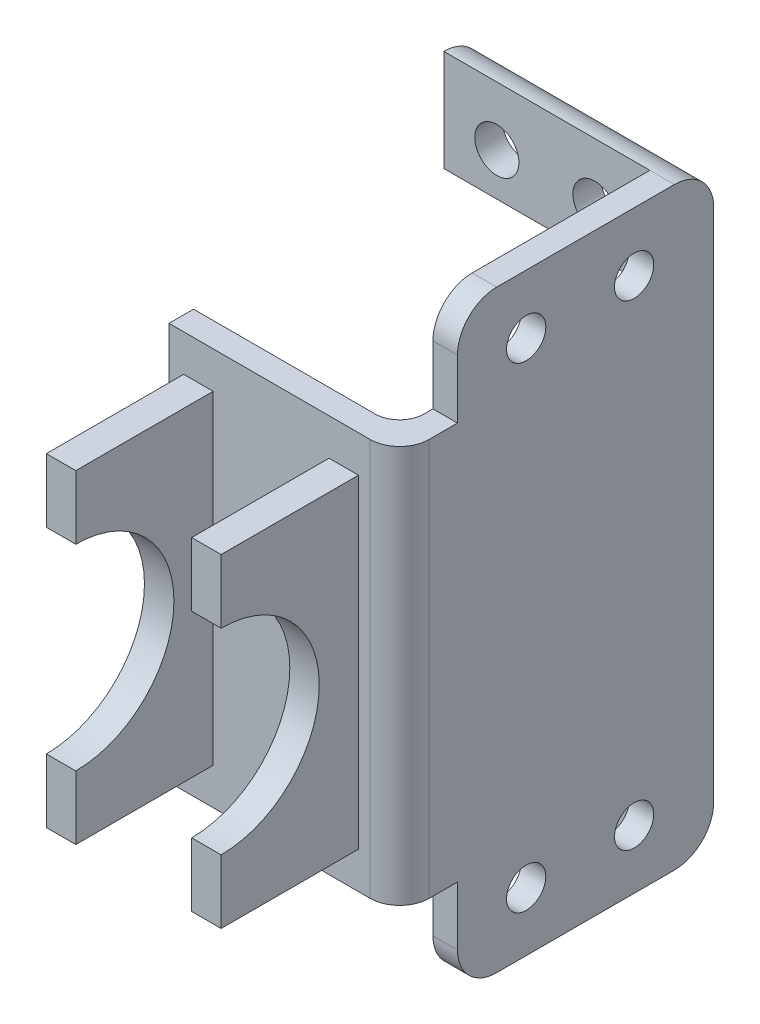
SolidWorks part; units mm, degrees
material "45"
ref_plane "Front Plane" through (0, 0, 0) normal (0, 0, 1) x (1, 0, 0)
ref_plane "Top Plane" through (0, 0, 0) normal (0, 1, 0) x (1, 0, 0)
ref_plane "Right Plane" through (0, 0, 0) normal (1, 0, 0) x (0, 0, -1)
sketch "Sketch2" plane through (0, 0, 0) normal (0, 0, 1) x (1, 0, 0)
  line L1 (10.5956, -30.2541) -> (-10.4044, -30.2541)
  line L2 (10.5956, -30.2541) -> (10.5956, 10.2459)
  line L3 (10.5956, 10.2459) -> (-10.4044, 10.2459)
  line L4 (-10.4044, -30.2541) -> (-10.4044, 10.2459)
  dimension "D1" = 21
  dimension "D2" = 40.5
extrude "Boss-Extrude1" add sketch "Sketch2" along normal blind 2.5
sketch "Sketch3" plane through (0, 0, 2.5) normal (0, 0, 1) x (1, 0, 0)
  line L0 (10.5956, -10.0041) -> (-49989.4044, -10.0041) construction
  line L1 (10.5956, -30.2541) -> (10.5956, 10.2459) construction
  line L2 (-10.4044, 10.2459) -> (-10.4044, -30.2541) construction
  line L3 (-5.9044, -26.5041) -> (-8.9044, -26.5041)
  line L4 (-5.9044, -26.5041) -> (-5.9044, 6.4959)
  line L5 (-5.9044, 6.4959) -> (-8.9044, 6.4959)
  line L6 (-8.9044, -26.5041) -> (-8.9044, 6.4959)
  line L7 (-5.9044, -26.5041) -> (-8.9044, 6.4959) construction
  line L8 (-5.9044, 6.4959) -> (-8.9044, -26.5041) construction
  line L9 (0, 0) -> (0, 50000) construction
  line L10 (5.9044, 6.4959) -> (8.9044, -26.5041) construction
  line L11 (5.9044, -26.5041) -> (8.9044, 6.4959) construction
  line L12 (8.9044, -26.5041) -> (8.9044, 6.4959)
  line L13 (5.9044, 6.4959) -> (8.9044, 6.4959)
  line L14 (5.9044, -26.5041) -> (5.9044, 6.4959)
  line L15 (5.9044, -26.5041) -> (8.9044, -26.5041)
  point P4 (10.5956, -10.0041)
  point P5 (-7.4044, -10.0041)
  point P19 (7.4044, -10.0041)
  dimension "D1" = 3
  dimension "D2" = 1.5
  dimension "D3" = 33
extrude "Boss-Extrude2" add sketch "Sketch3" along normal blind 14
sketch "Sketch4" plane through (8.9044, 0, 0) normal (1, 0, 0) x (0, 0, -1)
  line L1 (-16.5, -10.0041) -> (-38.1987, -10.0041) construction
  line L2 (-16.5, -26.5041) -> (-16.5, 6.4959) construction
  circle A0 centre (-16.5, -10.0041) radius 10
  dimension "D1" = 20
  dimension "D2" = 0
extrude "Cut-Extrude1" cut sketch "Sketch4" against normal through all
ref_plane "Plane1" through (0, -10.0041, 0) normal (0, 1, 0) x (1, 0, 0)
sketch "Sketch5" plane through (0, -10.0041, 0) normal (0, 1, 0) x (1, 0, 0)
  line L0 (10.5956, 0) -> (10.5956, 29.5)
  line L1 (10.5956, 29.5) -> (13.0956, 29.5)
  line L2 (13.0956, 29.5) -> (13.0956, -2.5)
  line L3 (13.0956, -2.5) -> (10.5956, -2.5)
  line L4 (10.5956, -2.5) -> (10.5956, 0)
  dimension "D1" = 2.5
  dimension "D2" = 32
extrude "Boss-Extrude3" add sketch "Sketch5" along normal mid plane 40.5
fillet "Fillet1" radius 3 1 edges at (13.0956, -10.0041, 2.5)
fillet "Fillet2" radius 2.5 1 edges
sketch "Sketch6" plane through (13.0956, 0, 0) normal (1, 0, 0) x (0, 0, -1)
  line L0 (29.5, -30.2541) -> (29.5, -36.2541)
  line L1 (25.5, -40.2541) -> (7.3954, -40.2541)
  line L2 (3.3954, -36.2541) -> (3.3954, -30.2541)
  line L3 (3.3954, -30.2541) -> (29.5, -30.2541)
  line L4 (3.3954, 10.2459) -> (29.5, 10.2459)
  line L5 (-6.5, -10.0041) -> (16.5374, -10.0041) construction
  line L6 (3.3954, 16.2459) -> (3.3954, 10.2459)
  line L7 (25.5, 20.2459) -> (7.3954, 20.2459)
  line L8 (29.5, 10.2459) -> (29.5, 16.2459)
  arc A0 (-16.5, -20.0041) -> (-16.5, -0.0041) centre (-16.5, -10.0041) ccw construction
  arc A1 (25.5, 20.2459) -> (29.5, 16.2459) centre (25.5, 16.2459) cw
  arc A2 (3.3954, 16.2459) -> (7.3954, 20.2459) centre (7.3954, 16.2459) cw
  arc A3 (7.3954, -40.2541) -> (3.3954, -36.2541) centre (7.3954, -36.2541) cw
  arc A4 (29.5, -36.2541) -> (25.5, -40.2541) centre (25.5, -36.2541) cw
  point P16 (29.5, 20.2459)
  point P19 (3.3954, 20.2459)
  point P22 (3.3954, -40.2541)
  point P25 (29.5, -40.2541)
  dimension "D3" = 4
  dimension "D1" = 10
  dimension "D2" = 26.1046
extrude "Boss-Extrude4" add sketch "Sketch6" against normal up to surface (2.5 mm away) up to face at (10.5956, -10.0041, -22.75)
sketch "Sketch7" plane through (13.0956, 0, 0) normal (1, 0, 0) x (0, 0, -1)
  line L0 (29.5, -10.0041) -> (0.5, -10.0041) construction
  line L1 (29.5, 16.2459) -> (29.5, -36.2541) construction
  line L2 (0.5, 10.2459) -> (0.5, -30.2541) construction
  line L3 (3.3954, -30.2541) -> (3.3954, -36.2541) construction
  line L4 (7.3954, -40.2541) -> (25.5, -40.2541) construction
  line L5 (10.3954, -34.2541) -> (21.3954, -34.2541) construction
  circle A0 centre (21.3954, -34.2541) radius 2
  circle A1 centre (10.3954, -34.2541) radius 2
  circle A2 centre (10.3954, 14.2459) radius 2
  circle A3 centre (21.3954, 14.2459) radius 2
  dimension "D1" = 4
  dimension "D2" = 4
  dimension "D3" = 11
  dimension "D4" = 7
  dimension "D5" = 6
extrude "Cut-Extrude2" cut sketch "Sketch7" against normal through all
sketch "Sketch9" plane through (10.5956, 0, 0) normal (-1, 0, 0) x (0, 0, 1)
  line L0 (-28.3284, -39.0826) -> (-28.3284, -29.9149)
  line L1 (-28.3284, -29.9149) -> (-25.5, -29.9149)
  line L2 (-25.5, -29.9149) -> (-25.5, -40.2541)
  arc A0 (-29.5, -36.2541) -> (-25.5, -40.2541) centre (-25.5, -36.2541) ccw construction
  arc A1 (-28.3284, -39.0826) -> (-25.5, -40.2541) centre (-25.5, -36.2541) ccw
extrude "Boss-Extrude5" add sketch "Sketch9" along normal blind 21
mirror "Mirror1" about plane through (0, -10.0041, 0) normal (0, 1, 0) of "Boss-Extrude5"
sketch "Sketch10" plane through (0, 0, -28.3284) normal (0, 0, -1) x (-1, 0, 0)
  line L0 (10.4044, -29.9149) -> (10.4044, -39.0826) construction
  line L2 (10.4044, -39.0826) -> (-10.5956, -39.0826) construction
  circle A0 centre (-5, -34.25) radius 2.25
  circle A1 centre (5, -34.25) radius 2.25
  dimension "D4" = 4.5
  dimension "D5" = 4.5
  dimension "D1" = 10
  dimension "D2" = 5.4044
  dimension "D3" = 4.8326
extrude "Cut-Extrude3" cut sketch "Sketch10" against normal blind 21
mirror "Mirror2" about plane through (0, -10.0041, 0) normal (0, 1, 0) of "Cut-Extrude3"
